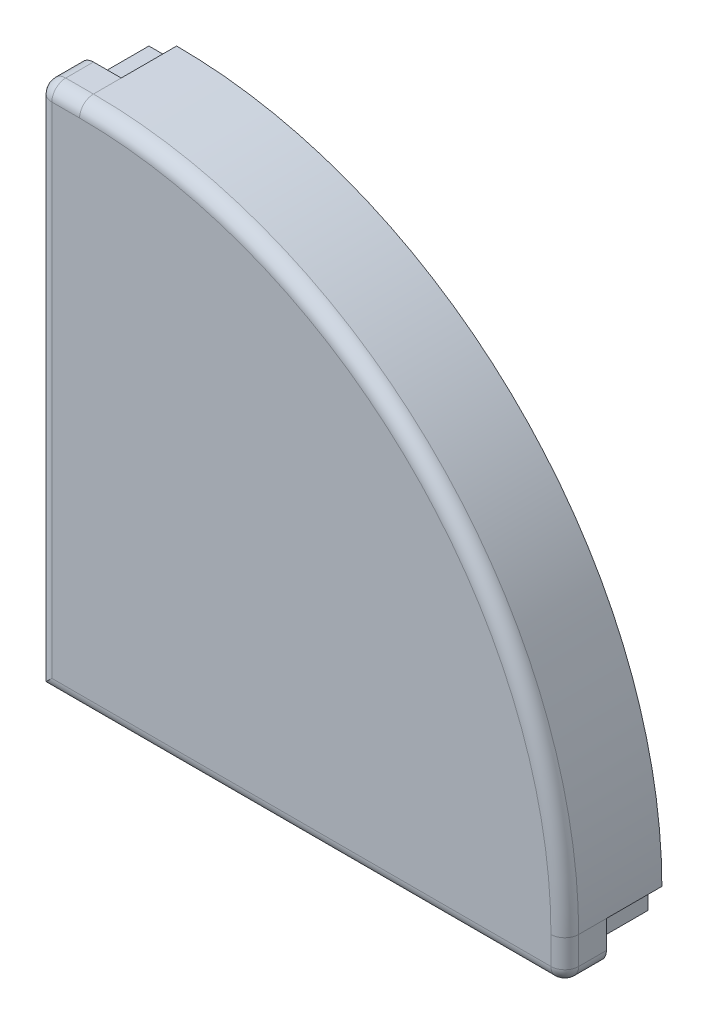
from build123d import *

# Parameters (mm, degrees)
BOSS_EXTRUDE1_DEPTH = 1.5
BOSS_EXTRUDE3_START = -2
BOSS_EXTRUDE3_DEPTH = 2
FILETE1_R           = 0.5


with BuildPart() as part:
    # Sketch1 → Boss-Extrude1 (new body)
    with BuildSketch(Plane.XY):
        with BuildLine():
            Line((0, 0), (0, 19))
            Line((0, 19), (1.5, 19))
            ThreePointArc((1.5, 19), (13.874368671, 13.874368671), (19, 1.5))
            Line((19, 1.5), (19, 0))
            Line((19, 0), (0, 0))
        make_face()
    extrude(amount=BOSS_EXTRUDE1_DEPTH)

    # Sketch2 → Boss-Extrude3 (add)
    # profile 1 of 2: a face of its own
    with BuildSketch(Plane.XY.offset(BOSS_EXTRUDE3_START)):
        with BuildLine():
            Line((1.5, 19), (1.5, 18.5))
            Line((1.5, 18.5), (0.5, 18.5))
            Line((0.5, 18.5), (0.5, 17.5))
            Line((0.5, 17.5), (1.5, 17.5))
            ThreePointArc((1.5, 17.5), (12.813708499, 12.813708499), (17.5, 1.5))
            Line((17.5, 1.5), (17.5, 0.5))
            Line((17.5, 0.5), (18.5, 0.5))
            Line((18.5, 0.5), (18.5, 1.5))
            Line((18.5, 1.5), (19, 1.5))
            ThreePointArc((19, 1.5), (13.874368671, 13.874368671), (1.5, 19))
        make_face()
    # profile 2 of 2: a face of its own
    with BuildSketch(Plane.XY.offset(BOSS_EXTRUDE3_START)):
        with BuildLine():
            Line((1.5, 16.5), (1.5, 0))
            Line((1.5, 0), (16.5, 0))
            Line((16.5, 0), (16.5, 1.5))
            ThreePointArc((16.5, 1.5), (12.106601718, 12.106601718), (1.5, 16.5))
        make_face()
        with BuildLine():
            Line((3, 14.916407865), (3, 1.5))
            Line((3, 1.5), (15, 1.5))
            ThreePointArc((15, 1.5), (11.562305899, 10.5), (3, 14.916407865))
        make_face(mode=Mode.SUBTRACT)
    extrude(amount=BOSS_EXTRUDE3_DEPTH)

    # Filete1
    filete1_edges = [part.edges().sort_by_distance(p)[0] for p in [
        (13.874368671, 13.874368671, 1.5),
        (0.75, 19, 1.5),
        (0, 9.5, 1.5),
        (9.5, 0, 1.5),
        (19, 0.75, 1.5),
        (0, 19, 0.75),
        (19, 0, 0.75),
    ]]
    fillet(filete1_edges, radius=FILETE1_R)


solid = part.part
